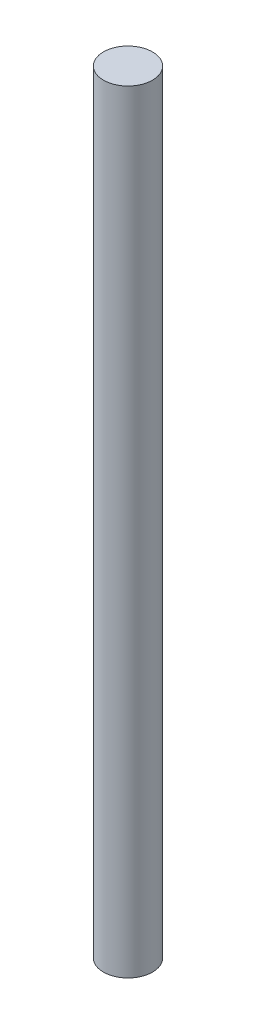
from build123d import *

# Parameters (mm, degrees)
SKETCH1_R           = 3.175
BOSS_EXTRUDE1_DEPTH = 100


with BuildPart() as part:
    # Sketch1 → Boss-Extrude1 (new body)
    with BuildSketch(Plane(origin=(0, 0, 0), x_dir=(1, 0, 0), z_dir=(0, 1, 0))):
        with Locations(Location((0, 0, 0), (0, 0, 270))):
            Circle(SKETCH1_R)
    extrude(amount=BOSS_EXTRUDE1_DEPTH)


solid = part.part
